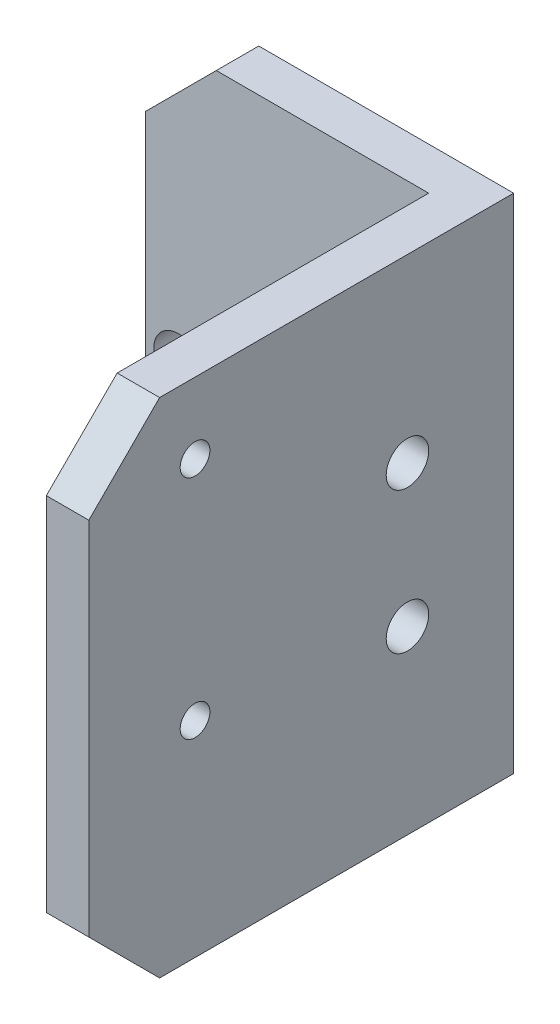
from build123d import *

# Parameters (mm, degrees)
SKETCH_1_W                = 60
SKETCH_1_H                = 71
EXTRUDE_1_DEPTH           = 6
HOLE_WIZARD_M5_1_D        = 4.2
HOLE_WIZARD_6_0_6_1_D     = 6
SKETCH_7_W                = 6
SKETCH_7_H                = 71
EXTRUDE_2_DEPTH           = 40
HOLE_WIZARD_7_0_7_1_D     = 7
HOLE_WIZARD_7_0_7_1_DEPTH = 15
HOLE_WIZARD_7_0_7_1_TIP   = 2.103012167
CUT_EXTRUDE_1_DEPTH       = 81.375680401
CHAMFER_1_SIZE            = 10


with BuildPart() as part:
    # 草图1 → 凸台-拉伸1 (new body)
    with BuildSketch(Plane(origin=(0, 0, 0), x_dir=(0, 0, -1), z_dir=(1, 0, 0))):
        Rectangle(SKETCH_1_W, SKETCH_1_H)
    extrude(amount=EXTRUDE_1_DEPTH)

    # M5 螺纹孔1 (through all)
    with Locations(Plane(origin=(6, 0, 0), x_dir=(0, 0, -1), z_dir=(1, 0, 0))):
        with Locations((-15, 25.5), (-15, -6.5)):
            Hole(HOLE_WIZARD_M5_1_D / 2)

    # Ø6.0 (6) 直径孔1 (through all)
    with Locations(Plane.ZY):
        with Locations((-15, 10), (-15, -10)):
            Hole(HOLE_WIZARD_6_0_6_1_D / 2)

    # 草图7 → 凸台-拉伸2 (add)
    with BuildSketch(Plane.ZY):
        with Locations((-27, 0)):
            Rectangle(SKETCH_7_W, SKETCH_7_H)
    extrude(amount=EXTRUDE_2_DEPTH)

    # Ø7.0 (7) 直径孔1
    with Locations(Plane(origin=(0, 0, -30), x_dir=(-1, 0, 0), z_dir=(0, 0, -1))):
        with Locations((20, 10)):
            Hole(HOLE_WIZARD_7_0_7_1_D / 2, depth=HOLE_WIZARD_7_0_7_1_DEPTH)
            with Locations((0, 0, -(HOLE_WIZARD_7_0_7_1_DEPTH + HOLE_WIZARD_7_0_7_1_TIP / 2))):  # 118° drill point
                Cone(0, HOLE_WIZARD_7_0_7_1_D / 2, HOLE_WIZARD_7_0_7_1_TIP, mode=Mode.SUBTRACT)

    # 草图10 → 切除-拉伸1 (cut, through all)
    with BuildSketch(Plane(origin=(0, 0, -30), x_dir=(-1, 0, 0), z_dir=(0, 0, -1))):
        with BuildLine():
            ThreePointArc((1.997955587, -5.105508828), (20, -13.5), (38.002044413, -5.105508828))
            ThreePointArc((38.002044413, -5.105508828), (37.570645496, -0.174596643), (32.639733311, -0.60599556))
            ThreePointArc((32.639733311, -0.60599556), (20, -6.5), (7.360266689, -0.60599556))
            ThreePointArc((7.360266689, -0.60599556), (2.429354504, -0.174596643), (1.997955587, -5.105508828))
        make_face()
    extrude(amount=-CUT_EXTRUDE_1_DEPTH, mode=Mode.SUBTRACT)

    # 倒角1
    chamfer_1_edges = [part.edges().sort_by_distance(p)[0] for p in [
        (-40, -35.5, -27),
        (-40, 35.5, -27),
        (3, -35.5, 30),
        (3, 35.5, 30),
    ]]
    chamfer(chamfer_1_edges, length=CHAMFER_1_SIZE)


solid = part.part
